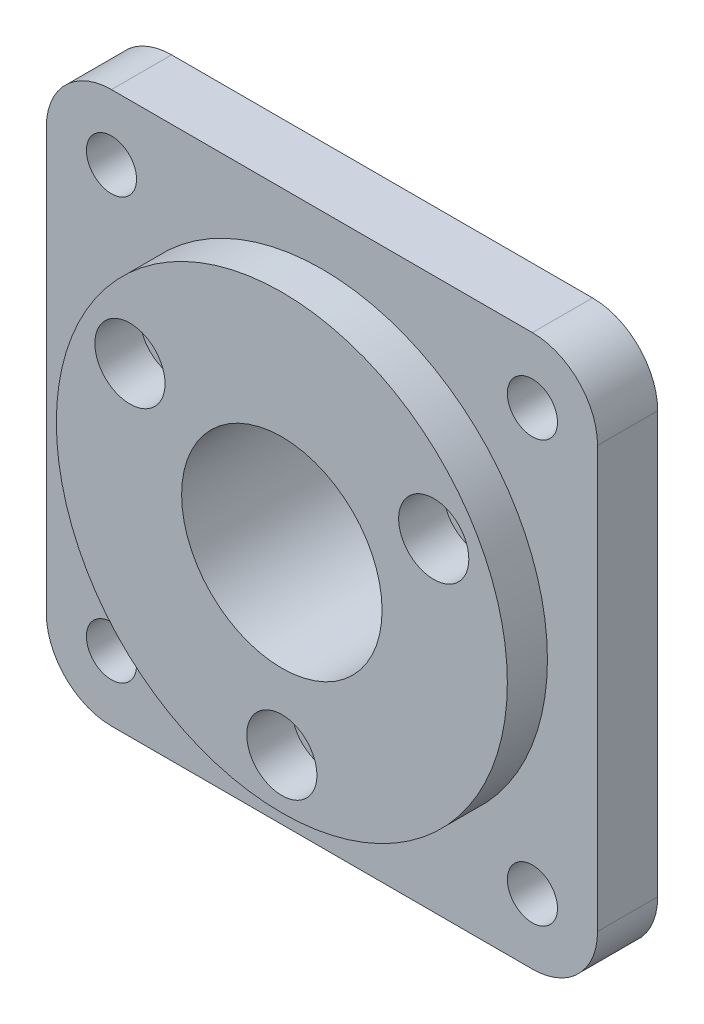
SolidWorks part; units mm, degrees
ref_plane "Front Plane" through (0, 0, 0) normal (0, 0, 1) x (1, 0, 0)
ref_plane "Top Plane" through (0, 0, 0) normal (0, 1, 0) x (1, 0, 0)
ref_plane "Right Plane" through (0, 0, 0) normal (1, 0, 0) x (0, 0, -1)
other "Configuration Table"
sketch "Sketch1" plane through (0, 0, 0) normal (0, 0, 1) x (1, 0, 0)
  line L1 (-42, -55) -> (42, -55)
  line L2 (-55, -42) -> (-55, 42)
  line L3 (-42, 55) -> (42, 55)
  line L4 (55, -42) -> (55, 42)
  line L5 (-55, -55) -> (55, 55) construction
  line L6 (-55, 55) -> (55, -55) construction
  arc A0 (42, -55) -> (55, -42) centre (42, -42) ccw
  arc A1 (-55, 42) -> (-42, 55) centre (-42, 42) cw
  arc A2 (-42, -55) -> (-55, -42) centre (-42, -42) cw
  arc A3 (42, 55) -> (55, 42) centre (42, 42) cw
  point P0 (0, 0)
  dimension "D3" = 13
  dimension "D1" = 110
  dimension "D2" = 110
extrude "Boss-Extrude1" add sketch "Sketch1" along normal blind 12
sketch "Sketch2" plane through (0, 0, 12) normal (0, 0, 1) x (1, 0, 0)
  circle A0 centre (42, 42) radius 5
  circle A1 centre (42, -42) radius 5
  circle A2 centre (-42, -42) radius 5
  circle A3 centre (-42, 42) radius 5
  point P11 (0, 0)
  dimension "D1" = 10
  dimension "D2" = 4
extrude "Cut-Extrude1" cut sketch "Sketch2" against normal blind 50
sketch "Sketch3" plane through (0, 0, 12) normal (0, 0, 1) x (1, 0, 0)
  circle A0 centre (0, 0) radius 45
  dimension "D1" = 90
extrude "Boss-Extrude2" add sketch "Sketch3" along normal blind 8
sketch "Sketch4" plane through (0, 0, 0) normal (0, 0, -1) x (-1, 0, 0)
  circle A0 centre (0, 0) radius 23.5
  dimension "D1" = 47
extrude "Boss-Extrude3" add sketch "Sketch4" along normal blind 9.8
sketch "Sketch6" plane through (0, 0, -9.8) normal (0, 0, -1) x (-1, 0, 0)
  circle A0 centre (0, 0) radius 20
  dimension "D1" = 40
extrude "Cut-Extrude2" cut sketch "Sketch6" against normal blind 80
sketch "Sketch7" plane through (0, 0, 20) normal (0, 0, 1) x (1, 0, 0)
  circle A0 centre (0, 0) radius 35 construction
  circle A1 centre (0, -35) radius 7
  dimension "D1" = 70
  dimension "D2" = 14
extrude "Cut-Extrude3" cut sketch "Sketch7" against normal blind 9
sketch "Sketch8" plane through (0, 0, 11) normal (0, 0, 1) x (1, 0, 0)
  circle A0 centre (0, -35) radius 4.5
  dimension "D1" = 9
extrude "Cut-Extrude4" cut sketch "Sketch8" against normal blind 801
pattern_circular "CirPattern1" count 3 over 360 about axis through (0, 0, 0) along (0, 0, 1) of "Cut-Extrude4", "Cut-Extrude3"
